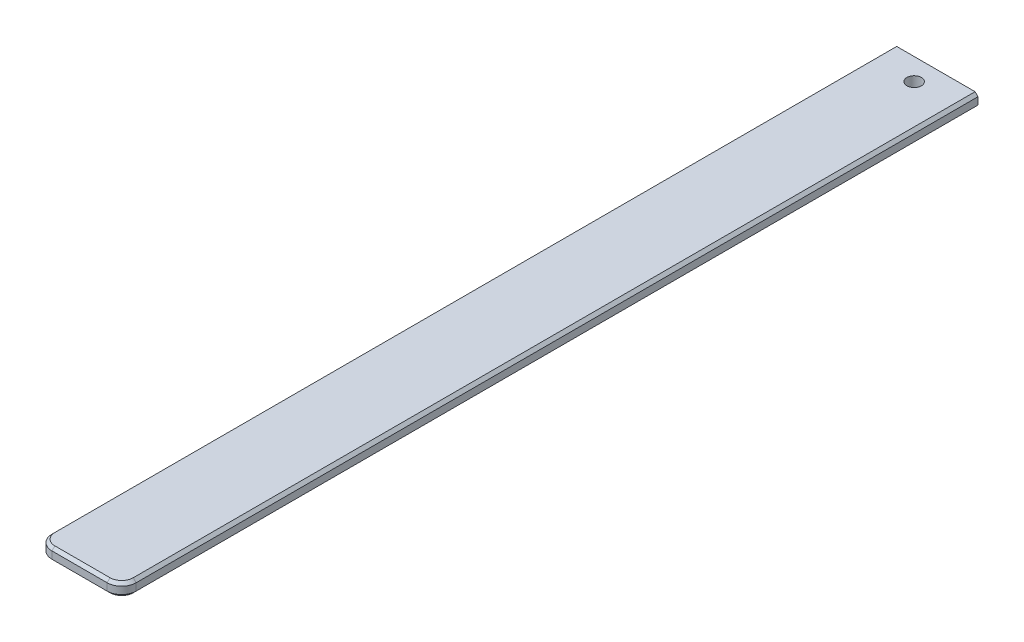
from build123d import *

# Parameters (mm, degrees)
SKETCH1_W           = 4.5
SKETCH1_H           = 3
BOSS_EXTRUDE1_DEPTH = 8
SKETCH2_W           = 2.9
SKETCH2_H           = 0.45
BOSS_EXTRUDE2_DEPTH = 26.5
FILLET1_R           = 0.5
CHAMFER1_SIZE       = 1
CHAMFER2_SIZE       = 0.1
SKETCH3_R           = 1.525
CUT_EXTRUDE1_DEPTH  = 2.1
SKETCH5_R           = 0.6
CUT_EXTRUDE2_DEPTH  = 2.1
CUT_EXTRUDE3_DEPTH  = 30.466082196
BOSS_EXTRUDE3_DEPTH = 3
SKETCH8_R           = 0.25
CUT_EXTRUDE4_DEPTH  = 3


with BuildPart() as part:
    # Sketch1 → Boss-Extrude1 (new body)
    with BuildSketch(Plane(origin=(0, 0, 0), x_dir=(1, 0, 0), z_dir=(0, 1, 0))):
        Rectangle(SKETCH1_W, SKETCH1_H)
    extrude(amount=BOSS_EXTRUDE1_DEPTH)

    # Sketch2 → Boss-Extrude2 (add)
    with BuildSketch(Plane.XY.offset(1.5)):
        with Locations((0, 0.425)):
            Rectangle(SKETCH2_W, SKETCH2_H)
    extrude(amount=BOSS_EXTRUDE2_DEPTH)

    # Fillet1
    fillet1_edges = [part.edges().sort_by_distance(p)[0] for p in [
        (1.45, 0.425, 28),
        (-1.45, 0.425, 28),
    ]]
    fillet(fillet1_edges, radius=FILLET1_R)

    # Chamfer1
    chamfer1_edges = [part.edges().sort_by_distance(p)[0] for p in [
        (0, 8, 1.5),
    ]]
    chamfer(chamfer1_edges, length=CHAMFER1_SIZE)

    # Chamfer2
    chamfer2_edges = [part.edges().sort_by_distance(p)[0] for p in [
        (0, 0.65, 28),
        (0, 0.2, 28),
        (1.45, 0.2, 14.5),
        (-1.45, 0.2, 14.5),
        (1.303553391, 0.2, 27.853553391),
        (-1.303553391, 0.2, 27.853553391),
        (-1.45, 0.65, 14.5),
        (1.45, 0.65, 14.5),
        (1.303553391, 0.65, 27.853553391),
        (-1.303553391, 0.65, 27.853553391),
    ]]
    chamfer(chamfer2_edges, length=CHAMFER2_SIZE)

    # Sketch3 → Cut-Extrude1 (cut)
    with BuildSketch(Plane.XY.offset(1.5)):
        with Locations((0, 3.825)):
            Circle(SKETCH3_R)
    extrude(amount=-CUT_EXTRUDE1_DEPTH, mode=Mode.SUBTRACT)

    # Sketch5 → Cut-Extrude2 (cut)
    with BuildSketch(Plane.XY.offset(-0.6)):
        with Locations((0, 3.825)):
            Circle(SKETCH5_R)
    extrude(amount=-CUT_EXTRUDE2_DEPTH, mode=Mode.SUBTRACT)

    # Sketch6 → Cut-Extrude3 (cut, through all)
    with BuildSketch(Plane(origin=(2.25, 0, 0), x_dir=(0, 0, -1), z_dir=(1, 0, 0))):
        Polygon((1.5, 8), (-0.5, 8), (-1.5, 7), (-1.5, 0), (1.5, 0), align=None)
    extrude(amount=-CUT_EXTRUDE3_DEPTH, mode=Mode.SUBTRACT)

    # Sketch7 → Boss-Extrude3 (add)
    with BuildSketch(Plane(origin=(0, 0, 1.5), x_dir=(-1, 0, 0), z_dir=(0, 0, -1))):
        Polygon((1.45, 0.55), (1.35, 0.65), (-1.35, 0.65), (-1.45, 0.55), (-1.45, 0.3), (-1.35, 0.2), (1.35, 0.2), (1.45, 0.3), align=None)
    extrude(amount=BOSS_EXTRUDE3_DEPTH)

    # Sketch8 → Cut-Extrude4 (cut)
    with BuildSketch(Plane.XZ.offset(-0.2)):
        with Locations(Location((0, -0.75, 0), (0, 0, 270))):
            Circle(SKETCH8_R)
    extrude(amount=-CUT_EXTRUDE4_DEPTH, mode=Mode.SUBTRACT)


solid = part.part
